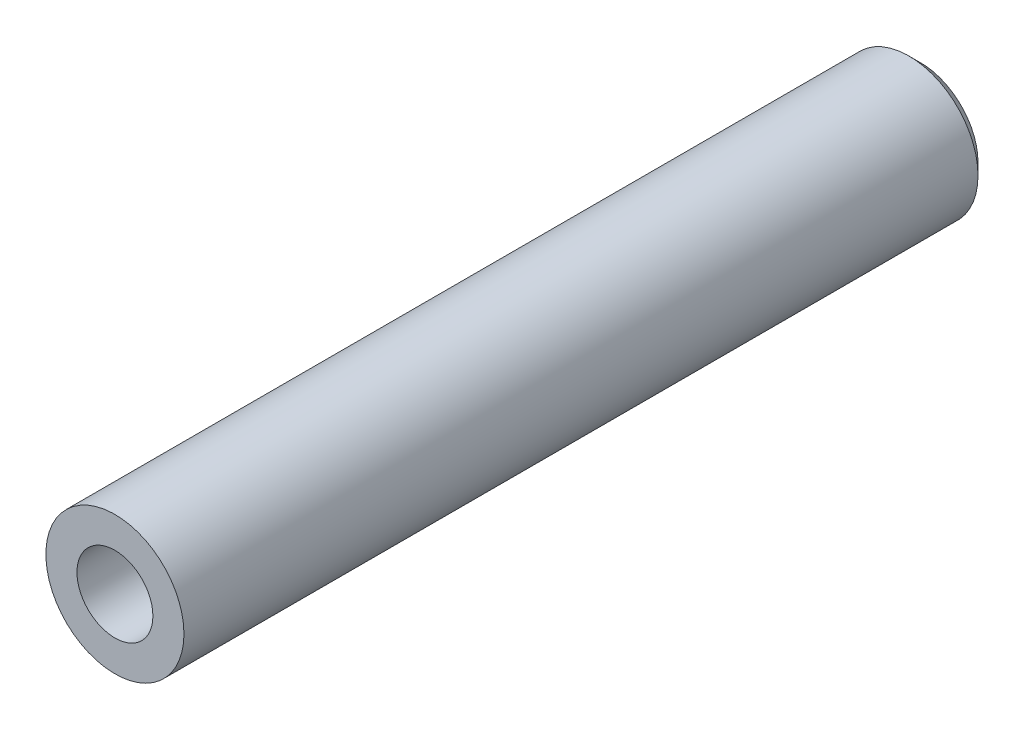
SolidWorks part; units mm, degrees
ref_plane "Front Plane" through (0, 0, 0) normal (0, 0, 1) x (1, 0, 0)
ref_plane "Top Plane" through (0, 0, 0) normal (0, 1, 0) x (1, 0, 0)
ref_plane "Right Plane" through (0, 0, 0) normal (1, 0, 0) x (0, 0, -1)
sketch "Sketch1" plane through (0, 0, 0) normal (0, 0, 1) x (1, 0, 0)
  circle A0 centre (0, 0) radius 3
  dimension "D1" = 6
extrude "Boss-Extrude1" add sketch "Sketch1" along normal mid plane 35
hole_wizard "M4 Tapped Hole1" positions "Sketch3" profile "Sketch2" tap size "M4" standard "Gb"
sketch "Sketch3" plane through (0, 0, 17.5) normal (0, 0, 1) x (1, 0, 0)
  point P0 (0, 0)
sketch "Sketch2" plane through (0, 0, 17.5) normal (1, 0, 0) x (0, -1, 0)
  line L0 (0, 0) -> (0, 11.0914)
  line L1 (0, 11.0914) -> (1.65, 10.1)
  line L2 (1.65, 10.1) -> (1.65, 0)
  line L5 (1.65, 0) -> (0, 0)
  line L10 (0, 11.0914) -> (-1.65, 10.1) construction
  line L11 (0, -6.35) -> (0, 107.95) construction
  dimension "螺纹孔钻头直径" = 3.3
  dimension "螺纹孔钻头深度" = 10.1
  dimension "导头角度" = 118
cosmetic thread "Hole Thread1" parameters "D1"=8, "D2"=4
chamfer "Chamfer1" distance 0.5 angle 45 1 edges at (3, 0, -17.5)
